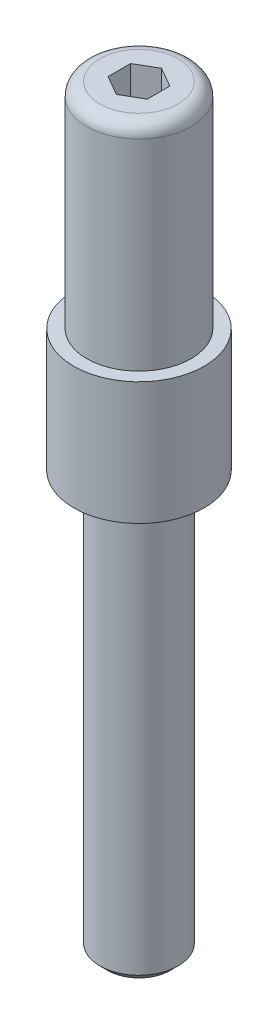
from build123d import *

# Parameters (mm, degrees)
CUT_EXTRUDE_1_DEPTH      = 3
CUT_EXTRUDE_1_DEPTH_BACK = 3


with BuildPart() as part:
    # 草图1 → 旋转1 (revolve)
    with BuildSketch(Plane.XY, mode=Mode.PRIVATE) as revolve_1_sk:
        with BuildLine():
            Line((0, 25.8), (3, 25.8))
            ThreePointArc((3, 25.8), (3.707106781, 25.507106781), (4, 24.8))
            Line((4, 24.8), (4, 9.4))
            Line((4, 9.4), (5, 9.4))
            Line((5, 9.4), (5, 0))
            Line((5, 0), (3, 0))
            Line((3, 0), (3, -31.3865))
            Line((3, -31.3865), (2.3865, -32))
            Line((2.3865, -32), (0, -32))
            Line((0, -32), (0, 25.8))
        make_face()
    revolve(revolve_1_sk.sketch.rotate(Axis((0, -32, 0), (0, 1, 0)), 270), axis=Axis((0, -32, 0), (0, 1, 0)))

    # 草图2 → 切除-拉伸1 (cut, two sides: drawn at the far end of the back side and taken through both)
    with BuildSketch(Plane(origin=(0, 25.8, 0), x_dir=(1, 0, 0), z_dir=(0, 1, 0)).offset(-CUT_EXTRUDE_1_DEPTH_BACK)):
        Polygon((-1.5, 0.866025404), (-1.5, -0.866025404), (0, -1.732050808), (1.5, -0.866025404), (1.5, 0.866025404), (0, 1.732050808), align=None)
    extrude(amount=CUT_EXTRUDE_1_DEPTH + CUT_EXTRUDE_1_DEPTH_BACK, mode=Mode.SUBTRACT)


solid = part.part
